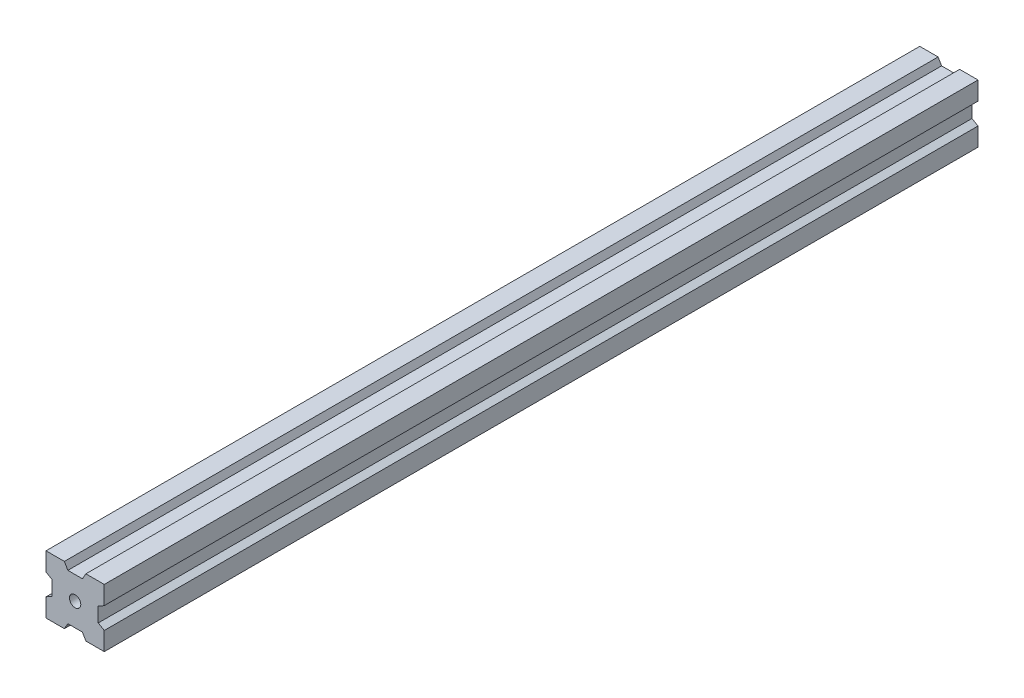
from build123d import *

# Parameters (mm, degrees)
SKETCH_1_W               = 20
SKETCH_1_H               = 20
SKETCH_1_R               = 1.94442565
EXTRUDE_1_DEPTH          = 150
CUT_EXTRUDE_1_DEPTH      = 301.333148354
PATTERN_CIRCULAR_1_COUNT = 4


with BuildPart() as part:
    # 草图1 → 凸台-拉伸1 (new, symmetric)
    with BuildSketch(Plane.XY):
        Rectangle(SKETCH_1_W, SKETCH_1_H)
        Circle(SKETCH_1_R, mode=Mode.SUBTRACT)
    extrude(amount=EXTRUDE_1_DEPTH, both=True)

    # 草图2 → 切除-拉伸1 (cut, symmetric)
    with BuildSketch(Plane.XY.offset(150)):
        Polygon((-32.933615203, 60.643738676), (-3.694439046, 10), (-2.5, 7.931170886), (2.5, 7.931170886), (3.694439046, 10), (32.933615203, 60.643738676), (32.933615203, 177.600443305), (-32.933615203, 177.600443305), align=None)
    cut_extrude_1 = extrude(amount=CUT_EXTRUDE_1_DEPTH, both=True, mode=Mode.SUBTRACT)

    # 阵列(圆周)1: 切除-拉伸1 ×4 about axis
    pattern_circular_1_axis = Axis((0, 0, 150), (0, 0, -1))
    for i in range(1, PATTERN_CIRCULAR_1_COUNT):
        add(cut_extrude_1.rotate(pattern_circular_1_axis, i * 360 / PATTERN_CIRCULAR_1_COUNT), mode=Mode.SUBTRACT)


solid = part.part
